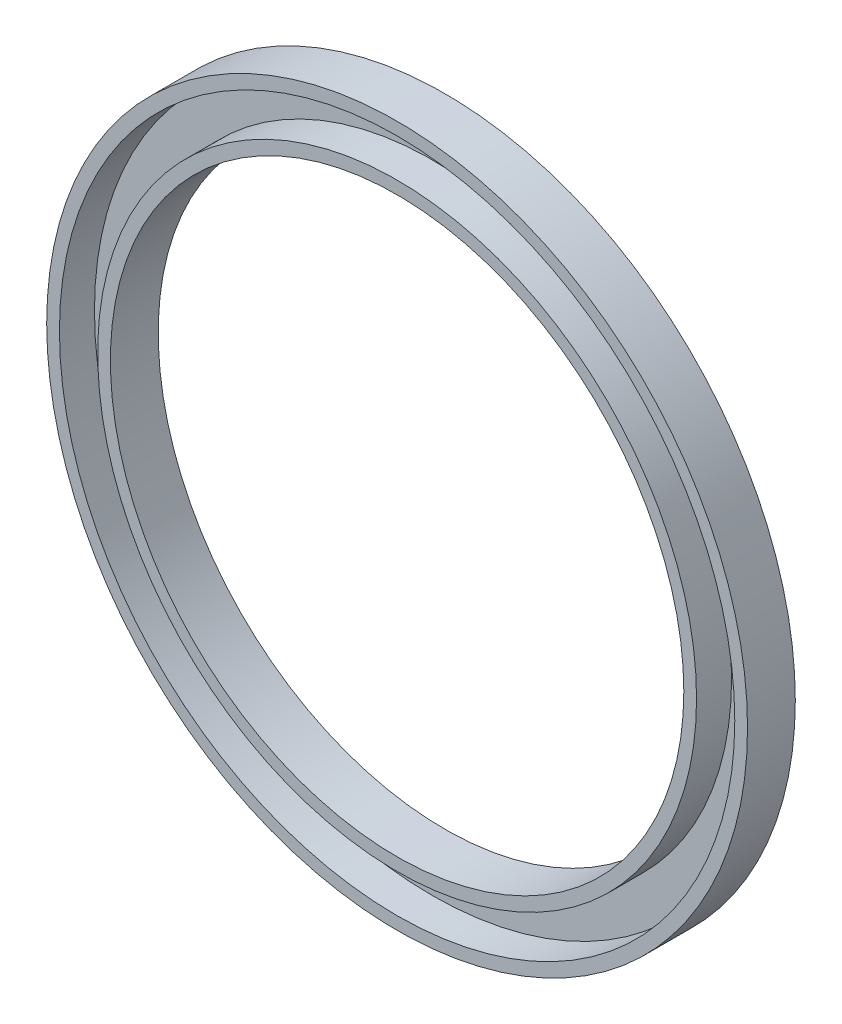
from build123d import *

# Parameters (mm, degrees)
SKETCH1_R           = 110
SKETCH1_R_2         = 90
BOSS_EXTRUDE1_DEPTH = 15
SHELL1_T            = -4


with BuildPart() as part:
    # Sketch1 → Boss-Extrude1 (new body)
    with BuildSketch(Plane.XY):
        Circle(SKETCH1_R)
        Circle(SKETCH1_R_2, mode=Mode.SUBTRACT)
    extrude(amount=BOSS_EXTRUDE1_DEPTH)

    # Shell1
    shell1_openings = [part.faces().sort_by_distance(p)[0] for p in [
        (-106.888730163, 0, 15),
    ]]
    offset(amount=SHELL1_T, openings=shell1_openings, kind=Kind.INTERSECTION)


solid = part.part
